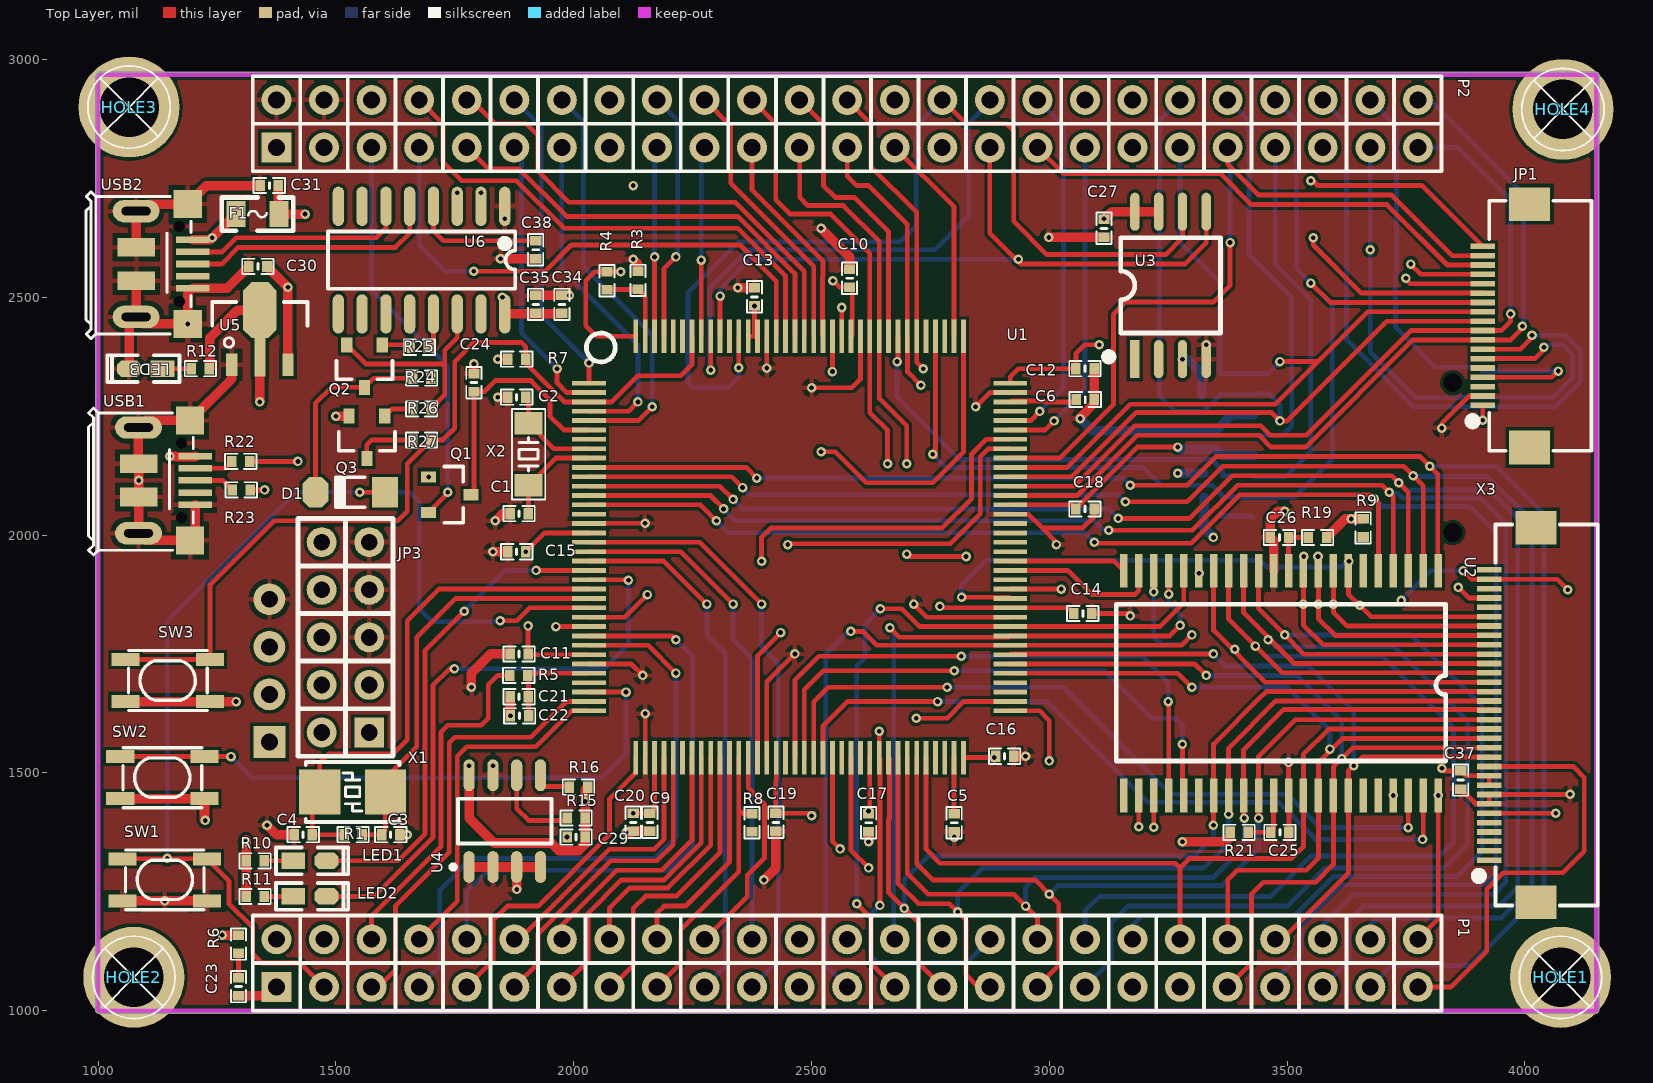
[diagram p0: Top Layer view]
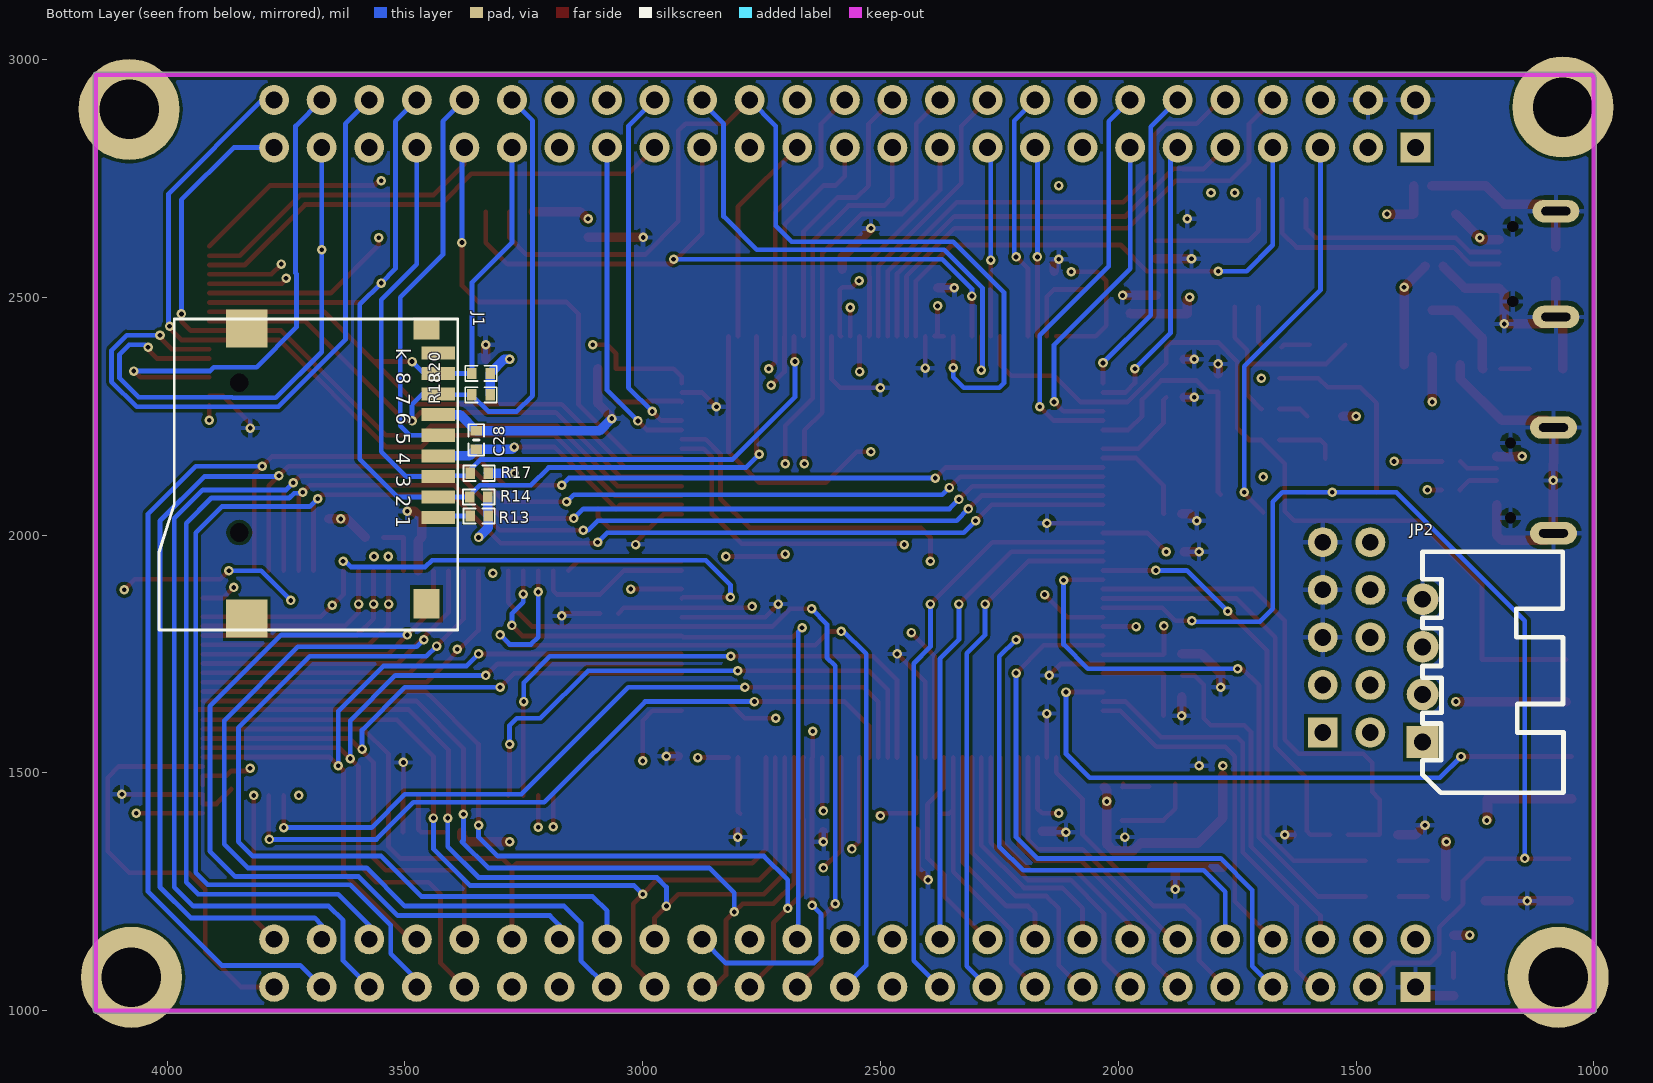
[diagram p1: Bottom Layer view, seen from below]
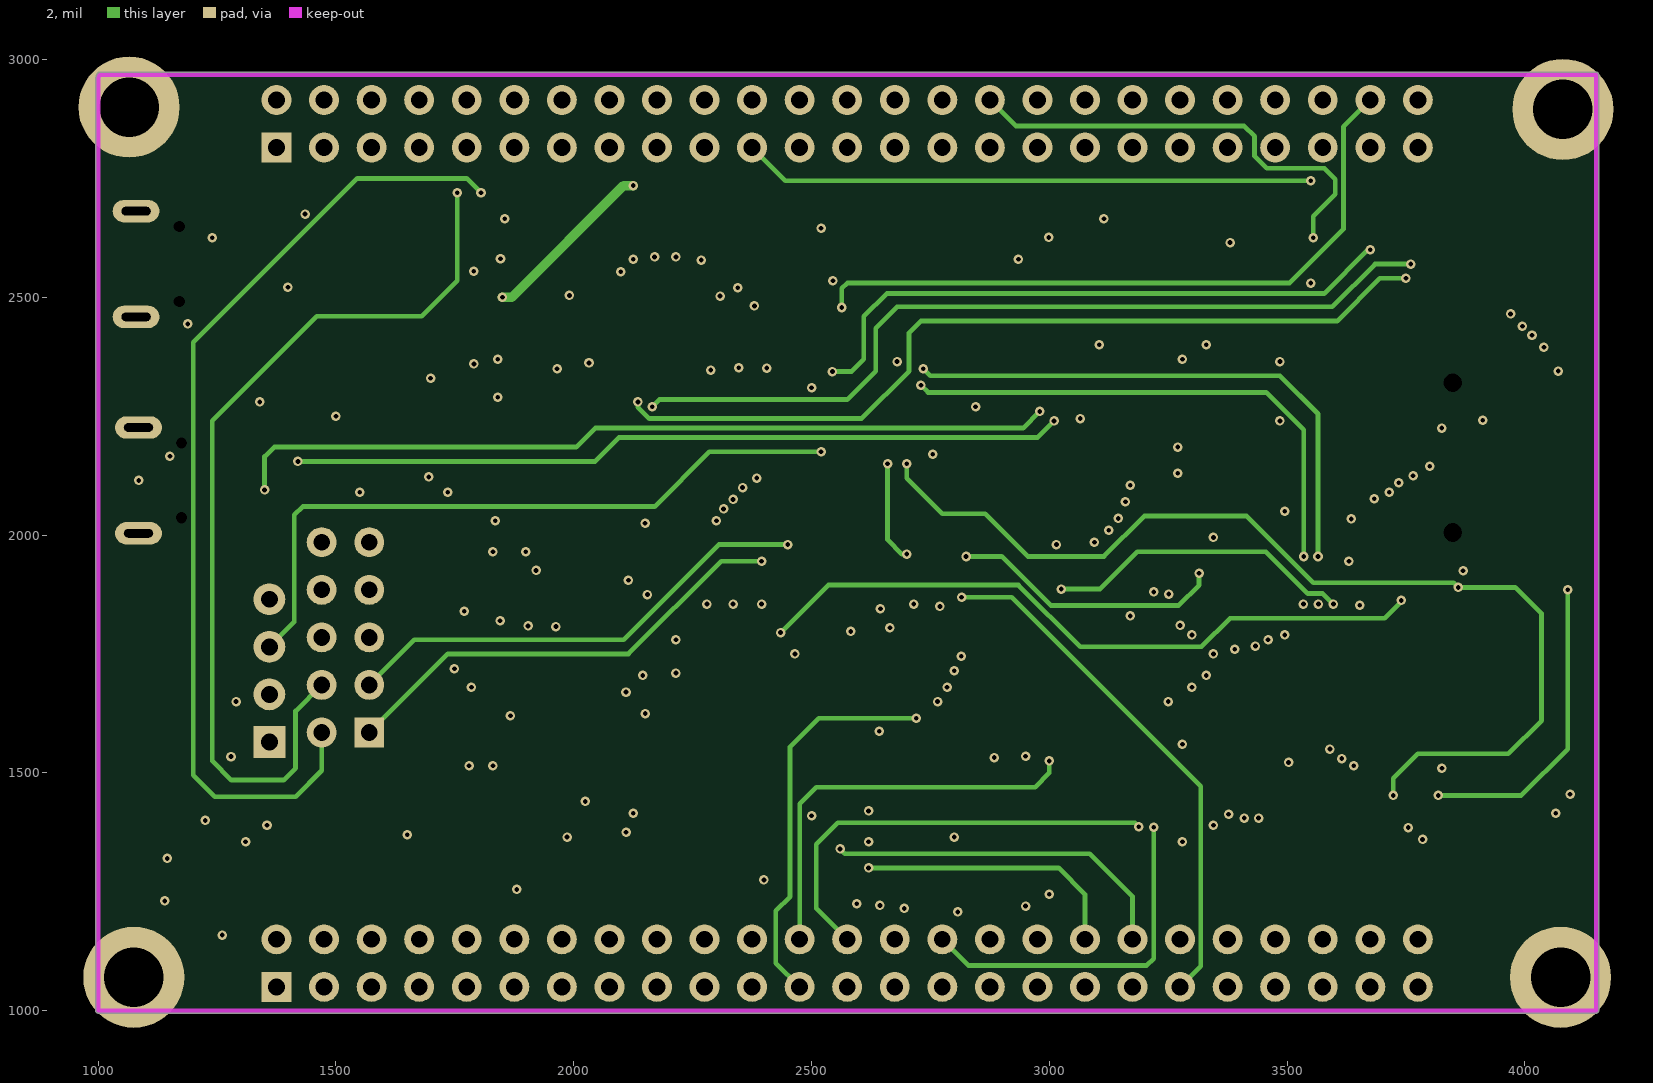
[diagram p2: 2]
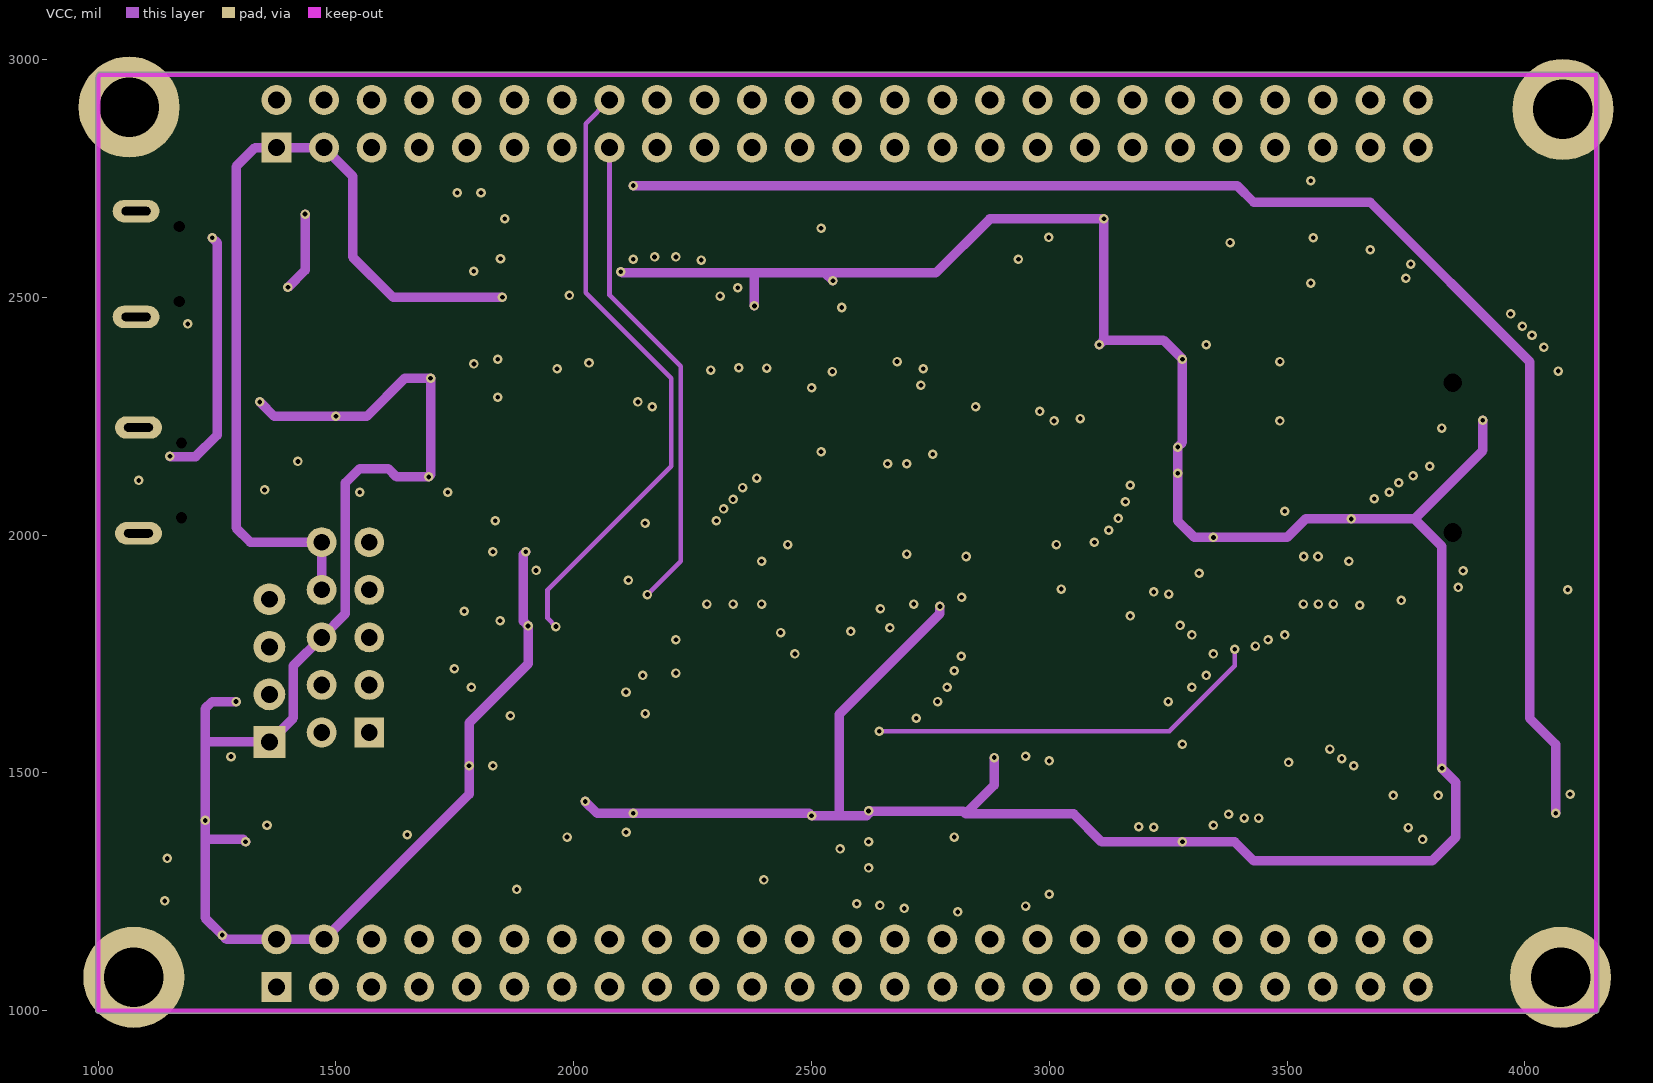
[diagram p3: VCC]
# Altium PCB MISC105440.PcbDoc (part 1 of 2)
Units mil, origin at the board's own origin, x right, y up, seen from the top; angles counter-clockwise.
Board outline 3160.03 x 1978.53 mil, 4 copper layers (Top Layer, 2, VCC, Bottom Layer), stack 30.634 mil thick; 91 components, 148 nets, 590 pads, 216 vias.

## Layer stack, top to bottom
Top Solder: solder mask 0.4, Solder Resist, Dk 3.5
Top Layer: signal copper 1.4
Dielectric 1: core 10, FR-4, Dk 4.2
2: signal copper 1.417
Dielectric 4: prepreg 5, Dk 4.2
VCC: signal copper 1.417
Dielectric 3: core 10, Dk 4.2
Bottom Layer: signal copper 1.4
Bottom Solder: solder mask 0.4, Solder Resist, Dk 3.5

## Board outline
1000,994.99 cw(c1000,1000) 994.99,1000 994.99,2960.15 cw(c1011.81,2960.15) 999.91,2972.05 cw(c1003.46,2968.5) 1003.46,2973.52 4149.61,2973.52 cw(c4149.61,2968.5) 4153.15,2972.05 cw(c4148.66,2967.55) 4155.02,2967.55 4155.02,1000 cw(c4150,1000) 4150,994.99

## Design rules (kind name [scope] priority, off if disabled: settings)
Clearance [All] p1: gap=7
HoleSize [All] p1: absolutevalues=TRUE maxlimit=99999 minlimit=1 maxpercent=80.000 minpercent=20.000
MinimumSolderMaskSliver [All] p1: minsoldermaskwidth=0
PolygonConnect [All] p1: connectstyle=Relief reliefconductorwidth=10 reliefentries=4 polygonreliefangle="90 Angle" airgapwidth=10
RoutingVias [All] p1: holewidth=28 width=50 viastyle="Through Hole" minholewidth=28 minwidth=50 maxholewidth=28 maxwidth=50
SilkToSilkClearance [All] p1: silktosilkclearance=0
SilkToSolderMaskClearance [IsPad] p1: minsilkscreentomaskgap=0 clearancetoexposedcopper=TRUE
SolderMaskExpansion [All] p1: expansion=4
Width [All] p1: maxlimit=30 minlimit=7 preferedwidth=7
26 further rules are at their usual default settings.

## Classes and differential pairs
component class Sheet1: C1 C2 C3 C4 C5 C6 C9 C10 C11 C12 C13 C14 C15 C16 C17 C18 C19 C20 C21 C22 C23 C24 JP1 JP2 P1 P2 Q1 R1 R3 R4 R5 R6 R7 R8 SW1 U1 X1 X2
component class Sheet2: C25 C26 C27 C28 C29 C30 C31 C34 C35 C37 C38 D1 F1 HOLE1 HOLE2 HOLE3 HOLE4 J1 JP3 LED1 LED2 LED3 Q2 Q3 R9 R10 R11 R12 R13 R14 R15 R16 R17 R18 R19 R20 R21 R22 R23 R24 R25 R26 R27 SW2 SW3 U2 U3 U4 U5 U6 USB1 USB2 X3

## Components (designator, comment, footprint, x,y, rotation, side; value= is the part's Value field where it differs from the comment)
C1 "10P" "C 0402" 1885,2045 r0 top
C2 "10P" "C 0402" 1880,2290 r0 top
C3 "22P" "C 0402" 1615,1370 r180 top
C4 "22P" "C 0402" 1431,1370 r0 top
C5 "225" "C 0402" 2800,1395 r270 top
C6 "225" "C 0402" 3075.59,2285 r0 top
C9 "104" "C 0402" 2160,1396 r90 top
C10 "104" "C 0402" 2580,2540 r270 top
C11 "104" "C 0402" 1885,1750 r0 top
C12 "104" "C 0402" 3075,2350 r180 top
C13 "104" "C 0402" 2380,2501 r270 top
C14 "104" "C 0402" 3070.59,1835 r180 top
C15 "104" "C 0402" 1880,1965 r0 top
C16 "104" "C 0402" 2906,1535 r180 top
C17 "104" "C 0402" 2620,1395 r90 top
C18 "104" "C 0402" 3075,2055 r180 top
C19 "104" "C 0402" 2425,1396 r90 top
C20 "104" "C 0402" 2125,1396 r90 top
C21 "10UF" "C 0402" 1885,1660 r180 top
C22 "104" "C 0402" 1886,1620 r180 top
C23 "104" "C 0402" 1295,1050.59 r270 top
C24 "104" "C 0402" 1790,2320.59 r270 top
C25 "10U" "C 0402" 3485,1375 r0 top
C26 "10U" "C 0402" 3484,1995 r180 top
C27 "104" "C 0402" 3115,2645 r270 top
C28 "104" "C 0402" 3350,2200 r270 bottom
C29 "104" "C 0402" 2005,1365 r0 top
C30 "22UF" "C 0402" 1336,2565 r0 top
C31 "104" "C 0402" 1360,2735 r0 top
C34 "10UF" "C 0402" 1975,2485 r90 top
C35 "104" "C 0402" 1920,2485 r90 top
C37 "104" "C 0402" 3865,1485 r90 top
C38 "104" "C 0402" 1920,2600 r90 top
D1 "1N4148" "MINI_MELF (LL34)" 1530,2090 r180 top
F1 "MSMD200-8V 2A" "FU 0805" 1335,2675 r0 top
HOLE1 "M3" "M3 5.4MM" 4075,1070 r0 top
HOLE2 "M3" "M3 5.4MM" 1075,1070 r0 top
HOLE3 "M3" "M3 5.4MM" 1065,2900 r0 top
HOLE4 "M3" "M3 5.4MM" 4080,2895 r0 top
J1 "TF_Card" "Micro SD" 3848.39,2162.76 r270 bottom
JP1 "FPC0.5-18P" "FPC0.5 2H-WS-18P" 4010,2440 r90 top
JP2 "SWD" XH2.54-WI-4P 1360,1715 r90 bottom
JP3 "Header 5X2" HDR2.54-LI-2x5P 1520,1785 r90 top
LED1 "Red" "LED 0603R" 1445,1314.74 r0 top
LED2 "Red" "LED 0603R" 1445,1240 r0 top
LED3 "Red" "LED 0603R" 1100,2350.26 r180 top
P1 "Header 25X2" HDR2.54-LI-2x25P 2325,1100 r0 top
P2 "Header 25X2" HDR2.54-LI-2x25P 2325,2865 r0 top
Q1 "BAT54C" SOT23-3L 1740,2085 r270 top
Q2 "SS8050" SOT23-3L 1560,2355 r180 top
Q3 "SS8550" SOT23-3L 1565,2205 r180 top
R1 "1M" "R 0402" 1536,1370 r180 top
R3 "0R" "R 0402" 2135,2535.59 r90 top
R4 "0R" "R 0402" 2070,2535 r90 top
R5 "10R" "R 0402" 1884.41,1705 r0 top
R6 "10K" "R 0402" 1295,1140 r90 top
R7 "10K" "R 0402" 1880,2370 r0 top
R8 "10K" "R 0402" 2375,1395 r90 top
R9 "10K" "R 0402" 3660,2015 r90 top
R10 "510" "R 0402" 1330,1315 r180 top
R11 "510" "R 0402" 1330,1240 r180 top
R12 "1K" "R 0402" 1215,2350 r0 top
R13 "47K" "R 0402" 3344,2040 r0 bottom
R14 "47K" "R 0402" 3345,2080 r0 bottom
R15 "4.7K" "R 0402" 2005,1405 r0 top
R16 "4.7K" "R 0402" 2010,1470 r0 top
R17 "47K" "R 0402" 3344,2130 r0 bottom
R18 "47K" "R 0402" 3340,2295 r0 bottom
R19 "2R" "R 0402" 3564,1995 r180 top
R20 "47K" "R 0402" 3340,2340 r0 bottom
R21 "2R" "R 0402" 3399,1375 r0 top
R22 "10R" "R 0402" 1300,2155 r0 top
R23 "10R" "R 0402" 1300.59,2095 r0 top
R24 "10K" "R 0402" 1680,2330 r180 top
R25 "1K" "R 0402" 1675.59,2395 r180 top
R26 "1K" "R 0402" 1680,2265 r180 top
R27 "1K" "R 0402" 1680,2200 r0 top
SW1 "3x6x5" "TSW SMD-3*4*2.5" 1140,1275 r0 top
SW2 "3x6x5" "TSW SMD-3*4*2.5" 1135,1490 r180 top
SW3 "3x6x5" "TSW SMD-3*4*2.5" 1146.42,1694.29 r180 top
U1 "STM32F407" "LQFP144 20X20_M" 2475,1975 r270 top
U2 "IS61LV51216" TSOP44_M 3817.93,1924.65 r270 top
U3 "W25Q128" SOP8W_L 3255,2525 r90 top
U4 "24C02C-E/ST" SOP8_L 1855,1398.54 r90 top
U5 "AS1117B" SOT89_L 1340,2370 r0 top
U6 "CH340G" SOP16 1855,2691.38 r270 top
USB1 "USB-DEVICE" USB-MICRO_B 1085,2115 r270 top
USB2 "USB-DEVICE" USB-MICRO_B 1080,2570 r270 top
X1 "8MHz" "OSC 5032-2P" 1535,1460 r180 top
X2 "32.768KHZ" "OSC 3215-2P" 1905,2170 r270 top
X3 "FPC0.5-32P" "FPC0.5 2H-WS-32P" 4023.31,1621.73 r90 top

## Footprints (in the part's own frame and the unit in brackets; to place one, negate y for a bottom-side part, rotate by r counter-clockwise, add the part's x,y. Pads: shape width x height; smd on the part's side, far side on the other; paste and mask are expansions set on the pad)
"C 0402" [mil] "无极性贴片电容"
  rect 20x23.62 smd mask+2: 1(-19,0) 2(19,0)
  silkscreen extent -33,-16 33,16, body extent -20,-10 20,10, height 20
"FPC0.5 2H-WS-18P" [mm] "长：13.2mm，宽：5.2mm，高：2mm"
  rect 1.8x2.2 smd: 0(-6.5,0) 0(6.5,0)
  rect 0.3x1.3 smd: 1(-4.25,2.497) 2(-3.75,2.497) 3(-3.25,2.497) 4(-2.75,2.497) 5(-2.25,2.497) 6(-1.75,2.497) 7(-1.25,2.497) 8(-0.75,2.497) 9(-0.25,2.497) 10(0.25,2.497) 11(0.75,2.497) 12(1.25,2.497) 13(1.75,2.497) 14(2.25,2.497) 15(2.75,2.497) 16(3.25,2.497) 17(3.75,2.497) 18(4.25,2.497)
  silkscreen extent -6.68,-3.3 6.68,3.23, body extent -6.6,-3.15 6.6,2.85, height 2
"FPC0.5 2H-WS-32P" [mm] "长：20.2mm，宽：5.2mm，高：2mm"
  rect 1.8x2.2 smd: 0(-10,0) 0(10,0)
  rect 0.3x1.3 smd: 1(-7.75,2.497) 2(-7.25,2.497) 3(-6.75,2.497) 4(-6.25,2.497) 5(-5.75,2.497) 6(-5.25,2.497) 7(-4.75,2.497) 8(-4.25,2.497) 9(-3.75,2.497) 10(-3.25,2.497) 11(-2.75,2.497) 12(-2.25,2.497) 13(-1.75,2.497) 14(-1.25,2.497) 15(-0.75,2.497) 16(-0.25,2.497) 17(0.25,2.497) 18(0.75,2.497) 19(1.25,2.497) 20(1.75,2.497) 21(2.25,2.497) 22(2.75,2.497) 23(3.25,2.497) 24(3.75,2.497) 25(4.25,2.497) 26(4.75,2.497) 27(5.25,2.497) 28(5.75,2.497) 29(6.25,2.497) 30(6.75,2.497) 31(7.25,2.497) 32(7.75,2.497)
  silkscreen extent -10.18,-3.3 10.17,3.23, body extent -10.1,-3.15 10.1,2.85, height 2
"FU 0805" [mil] "贴片保险丝"
  rect 40x55 smd: 1(-45,0) 2(45,0)
  silkscreen extent -75,-35 75,35, body extent -39,-24 39,24, height 20
HDR2.54-LI-2x5P [mm] "双排排针，5x2脚"
  rect 1.6x1.6 hole 0.9: 1(-5.08,-1.27)
  round 1.6 hole 0.9: 2(-5.08,1.27) 3(-2.54,-1.27) 4(-2.54,1.27) 5(0,-1.27) 6(0,1.27) 7(2.54,-1.27) 8(2.54,1.27) 9(5.08,-1.27) 10(5.08,1.27)
  silkscreen extent -6.35,-2.54 6.35,2.54, body extent -6.35,-2.54 6.35,2.54, height 8.5
HDR2.54-LI-2x25P [mm] "双排排针，25x2脚"
  rect 1.6x1.6 hole 0.9: 1(-24.13,-1.27)
  round 1.6 hole 0.9: 2(-24.13,1.27) 3(-21.59,-1.27) 4(-21.59,1.27) 5(-19.05,-1.27) 6(-19.05,1.27) 7(-16.51,-1.27) 8(-16.51,1.27) 9(-13.97,-1.27) 10(-13.97,1.27) 11(-11.43,-1.27) 12(-11.43,1.27) 13(-8.89,-1.27) 14(-8.89,1.27) 15(-6.35,-1.27) 16(-6.35,1.27) 17(-3.81,-1.27) 18(-3.81,1.27) 19(-1.27,-1.27) 20(-1.27,1.27) 21(1.27,-1.27) 22(1.27,1.27) 23(3.81,-1.27) 24(3.81,1.27) 25(6.35,-1.27) 26(6.35,1.27) 27(8.89,-1.27) 28(8.89,1.27) 29(11.43,-1.27) 30(11.43,1.27) 31(13.97,-1.27) 32(13.97,1.27) 33(16.51,-1.27) 34(16.51,1.27) 35(19.05,-1.27) 36(19.05,1.27) 37(21.59,-1.27) 38(21.59,1.27) 39(24.13,-1.27) 40(24.13,1.27) 41(26.67,-1.27) 42(26.67,1.27) 43(29.21,-1.27) 44(29.21,1.27) 45(31.75,-1.27) 46(31.75,1.27) 47(34.29,-1.27) 48(34.29,1.27) 49(36.83,-1.27) 50(36.83,1.27)
  silkscreen extent -25.4,-2.54 38.1,2.54, body extent -25.4,-2.54 38.1,2.54, height 8.5
"LED 0603R" [mil] "红色0603LED"
  rect 50x35 smd: 1(-35,0.26)
  oct 50x35 smd: 2(35,0.26)
  silkscreen extent -71,-28 81,28, body extent -31,-16 31,16, height 18
"LQFP144 20X20_M" [mm] "144脚，体宽20x20mm，脚距0.5mm"
  rect 0.254x1.8 smd: 1(-8.75,-11.25) 2(-8.25,-11.25) 3(-7.75,-11.25) 4(-7.25,-11.25) 5(-6.75,-11.25) 6(-6.25,-11.25) 7(-5.75,-11.25) 8(-5.25,-11.25) 9(-4.75,-11.25) 10(-4.25,-11.25) 11(-3.75,-11.25) 12(-3.25,-11.25) 13(-2.75,-11.25) 14(-2.25,-11.25) 15(-1.75,-11.25) 16(-1.25,-11.25) 17(-0.75,-11.25) 18(-0.25,-11.25) 19(0.25,-11.25) 20(0.75,-11.25) 21(1.25,-11.25) 22(1.75,-11.25) 23(2.25,-11.25) 24(2.75,-11.25) 25(3.25,-11.25) 26(3.75,-11.25) 27(4.25,-11.25) 28(4.75,-11.25) 29(5.25,-11.25) 30(5.75,-11.25) 31(6.25,-11.25) 32(6.75,-11.25) 33(7.25,-11.25) 34(7.75,-11.25) 35(8.25,-11.25) 36(8.75,-11.25) 73(8.75,11.25) 74(8.25,11.25) 75(7.75,11.25) 76(7.25,11.25) 77(6.75,11.25) 78(6.25,11.25) 79(5.75,11.25) 80(5.25,11.25) 81(4.75,11.25) 82(4.25,11.25) 83(3.75,11.25) 84(3.25,11.25) 85(2.75,11.25) 86(2.25,11.25) 87(1.75,11.25) 88(1.25,11.25) 89(0.75,11.25) 90(0.25,11.25) 91(-0.25,11.25) 92(-0.75,11.25) 93(-1.25,11.25) 94(-1.75,11.25) 95(-2.25,11.25) 96(-2.75,11.25) 97(-3.25,11.25) 98(-3.75,11.25) 99(-4.25,11.25) 100(-4.75,11.25) 101(-5.25,11.25) 102(-5.75,11.25) 103(-6.25,11.25) 104(-6.75,11.25) 105(-7.25,11.25) 106(-7.75,11.25) 107(-8.25,11.25) 108(-8.75,11.25)
  rect 1.8x0.254 smd: 37(11.25,-8.75) 38(11.25,-8.25) 39(11.25,-7.75) 40(11.25,-7.25) 41(11.25,-6.75) 42(11.25,-6.25) 43(11.25,-5.75) 44(11.25,-5.25) 45(11.25,-4.75) 46(11.25,-4.25) 47(11.25,-3.75) 48(11.25,-3.25) 49(11.25,-2.75) 50(11.25,-2.25) 51(11.25,-1.75) 52(11.25,-1.25) 53(11.25,-0.75) 54(11.25,-0.25) 55(11.25,0.25) 56(11.25,0.75) 57(11.25,1.25) 58(11.25,1.75) 59(11.25,2.25) 60(11.25,2.75) 61(11.25,3.25) 62(11.25,3.75) 63(11.25,4.25) 64(11.25,4.75) 65(11.25,5.25) 66(11.25,5.75) 67(11.25,6.25) 68(11.25,6.75) 69(11.25,7.25) 70(11.25,7.75) 71(11.25,8.25) 72(11.25,8.75) 109(-11.25,8.75) 110(-11.25,8.25) 111(-11.25,7.75) 112(-11.25,7.25) 113(-11.25,6.75) 114(-11.25,6.25) 115(-11.25,5.75) 116(-11.25,5.25) 117(-11.25,4.75) 118(-11.25,4.25) 119(-11.25,3.75) 120(-11.25,3.25) 121(-11.25,2.75) 122(-11.25,2.25) 123(-11.25,1.75) 124(-11.25,1.25) 125(-11.25,0.75) 126(-11.25,0.25) 127(-11.25,-0.25) 128(-11.25,-0.75) 129(-11.25,-1.25) 130(-11.25,-1.75) 131(-11.25,-2.25) 132(-11.25,-2.75) 133(-11.25,-3.25) 134(-11.25,-3.75) 135(-11.25,-4.25) 136(-11.25,-4.75) 137(-11.25,-5.25) 138(-11.25,-5.75) 139(-11.25,-6.25) 140(-11.25,-6.75) 141(-11.25,-7.25) 142(-11.25,-7.75) 143(-11.25,-8.25) 144(-11.25,-8.75)
  silkscreen extent -11.43,-11.39 -9.88,-9.84, body extent -11,-11 11,11, height 1.45
"M3 5.4MM" [mm] "M3螺丝孔，"
  round 5.4 hole 3.175: 0(0,0)
  silkscreen extent -2.2,-2.2 2.2,2.2
"Micro SD" [mm]
  round 0.85 hole 1 unplated: 0(-4,0) 0(4,0)
  rect 0.7x1.8 smd: 1(3.2,10.627) 2(2.1,10.627) 3(1,10.627) 4(-0.1,10.627) 5(-1.2,10.627) 6(-2.3,10.627) 7(-3.4,10.627) 8(-4.5,10.627) 9(-5.6,10.627)
  rect 2.032x2.2 smd: 10(-6.9,0.4) 10(8.6,0.4)
  rect 1.2x1.4 smd: 10(-6.9,10)
  rect 1.6x1.4 smd: 10(7.8,10)
  silkscreen extent -7.4,-4.28 9.2,11.67, body extent -7.05,-4 8.95,11.25, height 2
"MINI_MELF (LL34)" [mm] "1.5*3.4mm(直径，脚距）"
  rect 1.37x1.62 smd: 1(-1.855,0)
  oct 1.37x1.62 smd: 2(1.855,0)
  silkscreen extent -0.76,-0.8 0.78,0.8, body extent -1.7,-0.75 1.7,0.75, height 1.5
"OSC 3215-2P" [mm] "3.2*1.5*0.6mm(长宽高)"
  rect 1.2x1.5 smd: 1(-1.65,0) 2(1.65,0)
  silkscreen extent -2.41,-0.89 2.41,0.89, body extent -1.6,-0.75 1.6,0.75, height 0.61
"OSC 5032-2P" [mm] "5mm*3.2mm*0.8mm(长*宽*高)"
  rect 2.2x2.4 smd: 1(-1.75,0) 2(1.75,0)
  silkscreen extent -2.5,-1.6 2.5,1.6, body extent -2.5,-1.6 2.5,1.6, height 0.86
"R 0402" [mil] "1/16W贴片电阻"
  rect 20x23.62 smd mask+2: 1(-19,0) 2(19,0)
  silkscreen extent -33,-16 33,16, body extent -20,-10 20,10, height 12
SOP8_L [mm] "SOIC, 8-Leads, Body 4.9x3.9mm, Pitch 1.27mm, IPC High Density"
  oval 1.7x0.6 smd: 1(-2.45,1.905) 2(-2.45,0.635) 3(-2.45,-0.635) 4(-2.45,-1.905) 5(2.45,-1.905) 6(2.45,-0.635) 7(2.45,0.635) 8(2.45,1.905)
  silkscreen extent -2.57,-2.5 1.2,2.88, body extent -2,-2.5 2,2.5, height 1.75
SOP8W_L [mil] "5.3*8.3*1.8mm（长宽高）"
  rect 80x19.68 smd: 1(-155,75)
  oval 80x19.68 smd: 2(-155,25) 3(-155,-25) 4(-155,-75) 5(155,-75) 6(155,-25) 7(155,25) 8(155,75)
  silkscreen extent -156,-105 100,136, body extent -155,-104 155,104, height 75
SOP16 [mm]
  oval 2.1x0.6 smd: 1(0,0) 2(0,-1.27) 3(0,-2.54) 4(0,-3.81) 5(0,-5.08) 6(0,-6.35) 7(0,-7.62) 8(0,-8.89) 9(5.75,-8.89) 10(5.75,-7.62) 11(5.75,-6.35) 12(5.75,-5.08) 13(5.75,-3.81) 14(5.75,-2.54) 15(5.75,-1.27) 16(5.75,0)
  silkscreen extent 1.35,-9.45 4.4,0.56, body extent -0.04,-9.45 5.97,0.56, height 1.9
SOT23-3L [mm] "3x1.3x1mm(长宽高)"
  rect 0.6x0.8 smd: 1(-0.95,-1.143) 2(0.95,-1.143) 3(0,1.125)
  silkscreen extent -1.5,-0.3 1.5,0.7, body extent -1.5,-1.2 1.5,1.2, height 1.05
SOT89_L [mm] "4.6x4.3x1.6mm(长宽高)"
  rect 0.6x1.2 smd: 1(-1.5,-0.303) 3(1.5,-0.303)
  rect 0.6x2.1 smd: 2(0,0.127)
  oct 1.8x3 smd: 2(0,2.616)
  silkscreen extent -2.54,0.64 2.54,3.05, body extent -2.31,-0.63 2.29,3.67, height 1.6
TSOP44_M [mm]
  rect 1.8x0.4 smd: 1(-0.009,0.001) 2(-0.009,-0.799) 3(-0.009,-1.599) 4(-0.009,-2.399) 5(-0.009,-3.199) 6(-0.009,-3.999) 7(-0.009,-4.799) 8(-0.009,-5.599) 9(-0.009,-6.399) 10(-0.009,-7.199) 11(-0.009,-7.999) 12(-0.009,-8.799) 13(-0.009,-9.599) 14(-0.009,-10.399) 15(-0.009,-11.199) 16(-0.009,-11.999) 17(-0.009,-12.799) 18(-0.009,-13.599) 19(-0.009,-14.399) 20(-0.009,-15.199) 21(-0.009,-15.999) 22(-0.009,-16.799) 23(11.991,-16.799) 24(11.991,-15.999) 25(11.991,-15.199) 26(11.991,-14.399) 27(11.991,-13.599) 28(11.991,-12.799) 29(11.991,-11.999) 30(11.991,-11.199) 31(11.991,-10.399) 32(11.991,-9.599) 33(11.991,-8.799) 34(11.991,-7.999) 35(11.991,-7.199) 36(11.991,-6.399) 37(11.991,-5.599) 38(11.991,-4.799) 39(11.991,-3.999) 40(11.991,-3.199) 41(11.991,-2.399) 42(11.991,-1.599) 43(11.991,-0.799) 44(11.991,0.001)
  silkscreen extent 1.77,-17.2 10.16,0.4, body extent 0.1,-17.55 11.86,0.66, height 1.3
"TSW SMD-3*4*2.5" [mm] "3*4*2.5mm"
  rect 1.5x0.7 smd: 1(-2.25,1.125) 1(2.25,1.125) 2(-2.25,-1.125) 2(2.25,-1.125)
  silkscreen extent -2.1,-1.6 2.1,1.6
USB-MICRO_B [mm] "micro型USB ，5.9*8.2*2.5mm"
  rect 0.35x1.8 smd: 1(-1.295,3.021) 2(-0.648,3.021) 3(0,3.021) 4(0.648,3.021) 5(1.295,3.021)
  rect 1.5x1.5 smd: 5(-3.2,2.754) 5(3.2,2.754)
  oval 1.2x2.5 hole 0.45 slot 1.55 at 90 deg: 5(-2.825,-0.006) 5(2.825,-0.006)
  round 0 hole 0.6 unplated: 5(-2,2.294) 5(2,2.294)
  rect 1x2 smd: 5(-0.889,0.01) 5(0.889,0.01)
  silkscreen extent -3.86,-2.67 3.99,2.92, body extent -4,-2.72 4,3.36, height 2.8
XH2.54-WI-4P [mm] "接插件，4P"
  rect 1.7x1.7 hole 0.9: 1(-3.81,0)
  round 1.7 hole 0.9: 2(-1.27,0) 3(1.27,0) 4(3.81,0)
  silkscreen extent -6.53,-7.53 6.35,0, body extent -6.31,-7.35 6.31,0.35, height 5.73

## Part data
C1 C2 C3 C4 C5 C6 C9 C10 C11 C12 C13 C14 C15 C16 C17 C18 C19 C20 C21 C22 C23 C24 C25 C26 C27 C28 C29 C30 C31 C34 C35 C38: library part C, "SMD capacitor"
C37: library part C, "Non-polar SMD capacitor"
D1: "Switching diode"
F1: library part FU, "SMD fuse"
HOLE1 HOLE2 HOLE3 HOLE4: "Copper pillar hole"
J1: "TF card socket"
JP1: library part FPC-18P, "FPC connector"
JP2: library part "Header 4", "4P connector"
JP3: "5*2P connector"
LED1 LED2 LED3: library part LED-SMD, "SMD LED"
P1 P2: "Header, 25-Pin, Dual row"
Q1: "SMD Schottky diode"
Q2: library part 8050-SMD, "RF amplifier, NPN type"
Q3: library part 8550-SMD, "RF amplifier, PNP type"
R1 R3 R4 R5 R6 R7 R8 R9 R10 R11 R12 R13 R14 R15 R16 R17 R18 R19 R20 R21 R22 R23 R24 R25 R26 R27: library part R, "SMD resistor"
SW1 SW2 SW3: library part "TSW 3x6", "3x6 tactile switch"
U2: "Static RAM"
U4: "2Kbit, 400kHz, 5V, I2C Serial EEPROM, 8-Pin TSSOP, Extended Temperature"
U5: library part AMS1117, "Three-terminal voltage regulator"
U6: "USB2UART"
USB1 USB2: library part USB-5P, "Micro USB receptacle"
X1 X2: library part XTAL-2P, "2-pin passive crystal oscillator"
X3: library part FPC-32P, "FPC connector"

## Via types
v1: diameter 20, hole 10, Top Layer to Bottom Layer, 216 vias

## Nets (pads, with @x,y where several pads share a name; then routed paths per layer and width w, separated by ;. In a path a pad name is that pad's centre, name@x,y a point inside that pad or via, vN(x,y) a via of type N, cw(c..) or ccw(c..) an arc to the next point about the centre after c; other vN are vias at no path point)
BOOT0: R7.2 R27.2 SW3.2 U1.3 U1.138 | length 1863.7
  Top Layer w10: SW3.2@1057.83,1738.58 SW3.2@1235,1738.58 1235,1895 1370,2030 1630,2030 1650,2050 1650,2150.22 1699,2199.22 R27.2@1699,2200 1725,2200 1750,2225 1750,2365 1790,2405 1890,2405 1899,2396 R7.2@1899,2370 1899,2361 1979.88,2280.12 U1.3@2032.09,2280.12 2080.12,2280.12 2135,2335 2225,2335 2248.62,2358.62 U1.138@2248.62,2417.91
BOOT1: P1.17 R8.2 U1.48 | length 585
  Top Layer w10: P1.17@2175,1050 2225,1100 2225,1170 2347.05,1292.05 2347.05,1422.95 ; U1.48@2347.05,1532.09 2347.05,1422.95 ; R8.2@2375,1414 2356,1414 2347.05,1422.95
CH340_D+: U6.5 USB2.3 | length 554.4
  Top Layer w10: USB2.3@1198.94,2570 1260,2570 1295,2605 1625,2605 1655,2635 U6.5@1655,2691.38 U6.5@1655,2706.38
CH340_D-: U6.6 USB2.2 | length 487.9
  Top Layer w10: USB2.2@1198.94,2595.5 1260.5,2595.5 1290,2625 1585,2625 1605,2645 U6.6@1605,2691.38 U6.6@1605,2706.38
DCMI_D0: JP1.8 P2.50 U1.96 | length 1834.9
  Top Layer w10: U1.96@2917.91,2083.27 3058.27,2083.27 3185,2210 3440.96,2210 3465.96,2185 3539.04,2185 3764.51,2410.47 JP1.8@3911.69,2410.47 3970.47,2410.47 3995,2435 v1(3995,2439)
  Bottom Layer w10: P2.50@3775,2915 3800,2915 3997,2718 3997,2437 v1(3995,2439)
DCMI_D1: JP1.9 P2.49 U1.97 | length 1708
  Top Layer w10: U1.97@2917.91,2102.95 3052.95,2102.95 3180,2230 3445,2230 3465,2210 3540,2210 3760.16,2430.16 JP1.9@3911.69,2430.16 3950.16,2430.16 3970,2450 v1(3970,2465)
  Bottom Layer w10: P2.49@3775,2815 3860,2815 3970,2705 v1(3970,2465)
DCMI_D2: J1.7 JP1.10 P2.40 R18.2 U1.98 | length 2110.7
  Top Layer w10: U1.98@2917.91,2122.64 3047.64,2122.64 3183,2258 3467,2258 v1(3485,2240) 3500,2240 3709.84,2449.84 JP1.10@3911.69,2449.84
  Bottom Layer w10: P2.40@3275,2915 3231.5,2871.5 3231.5,2293.5 3265,2260 3324.78,2260 3359,2294.22 R18.2@3359,2295 3428.39,2295 J1.7@3430,2296.61 3463.39,2296.61 3485,2275 v1(3485,2240)
DCMI_D3: J1.8 JP1.11 P2.39 R20.2 U1.99 | length 1855.4
  Top Layer w10: U1.99@2917.91,2142.32 3037.32,2142.32 3170,2275 3475,2275 3564.76,2364.76 ; v1(3485,2365) 3564.53,2365 3564.76,2364.76 ; JP1.11@3911.69,2469.53 3669.53,2469.53 3564.76,2364.76
  Bottom Layer w10: P2.39@3275,2815 3275,2615 3359,2531 R20.2@3359,2340 3359.08,2339.92 J1.8@3430,2339.92 3459.92,2339.92 v1(3485,2365)
DCMI_D4: J1.2 JP1.12 P2.44 R14.2 U1.112 | length 2345.8
  Top Layer w10: v1(2755,2170) 2760.43,2164.57 U1.112@2760.43,2417.91 ; v1(3550,2530) 3590.79,2489.21 JP1.12@3911.69,2489.21
  Bottom Layer w10: v1(2755,2170) 2783,2142 3198,2142 3235,2105 3342.78,2105 3364,2083.78 R14.2@3364,2080 ; 3375.08,2080.08 J1.2@3430,2080.08 3515.08,2080.08 3595,2160 3595,2485 v1(3550,2530) 3520,2560 3520,2870.01 P2.44@3475,2915
DCMI_D5: JP1.13 P2.32 U1.136 | length 2490.9
  Top Layer w10: v1(2287.99,2347.01) U1.136@2287.99,2417.91 ; v1(3555,2625) 3555,2610 3656.1,2508.9 JP1.13@3911.69,2508.9
  2 w10: P2.32@2875,2915 2930,2860 3410,2860 3431.51,2838.49 3431.51,2796.99 3456.99,2771.51 3578.49,2771.51 3601.5,2748.5 3601.5,2716.5 3555,2670 v1(3555,2625)
  Bottom Layer w10: v1(2287.99,2347.01) 2285.68,2349.32 2285.68,2519.72 2365.96,2600 2760,2600 2830,2670 2830,2865 2875,2910 P2.32@2875,2915
DCMI_D6: JP1.14 P2.13 U1.4 | length 2685.4
  Top Layer w10: U1.4@2032.09,2260.43 2115.43,2260.43 v1(2135,2280) ; v1(3750,2540) 3750,2537.16 3758.58,2528.58 JP1.14@3911.69,2528.58
  2 w10: v1(2135,2280) 2135,2268.89 2158.89,2245 2605,2245 2705,2345 2705,2425 2730,2450 3605,2450 3695,2540 v1(3750,2540)
  Bottom Layer w10: P2.13@1975,2815 1975,2560 2135,2400 v1(2135,2280)
DCMI_D7: JP1.15 P2.14 U1.5 | length 2802.1
  Top Layer w10: U1.5@2032.09,2240.75 2135.75,2240.75 v1(2165,2270) ; v1(3760,2570) 3760,2568.89 3780.62,2548.27 JP1.15@3911.69,2548.27
  2 w10: v1(2165,2270) 2180,2285 2575,2285 2635,2345 2635,2435 2680,2480 3595,2480 3685,2570 v1(3760,2570)
  Bottom Layer w10: P2.14@1975,2915 2020,2870 2020,2565 2165,2420 v1(2165,2270)
DCMI_HREF: P1.12 U1.40 | length 573.9
  Top Layer w10: P1.12@1875,1150 1885,1150 2074.57,1339.57 2169.57,1339.57 2189.57,1359.57 U1.40@2189.57,1532.09
DCMI_PCLK: JP1.16 P2.33 | length 1039
  Top Layer w10: P2.33@2975,2815 3030,2760 3360,2760 3425,2695 3710,2695 3837.05,2567.95 JP1.16@3911.69,2567.95
DCMI_PWDN: JP1.18 P2.21 U1.124 | length 2082.6
  Top Layer w10: P2.21@2375,2815 2375,2725 2524.21,2575.79 2524.21,2545.33 2523,2544.11 2523,2419.13 U1.124@2524.21,2417.91 ; v1(3550,2745) 3555,2745 3565,2735 3784.02,2735 JP1.18@3911.69,2607.32
  2 w10: P2.21@2375,2815 2445,2745 v1(3550,2745)
DCMI_RESET: JP1.7 P2.46 | length 1402.9
  Top Layer w10: JP1.7@3911.69,2390.79 3990.79,2390.79 4020,2420 v1(4015,2420)
  Bottom Layer w10: P2.46@3575,2915 3625,2865.01 3625,2410.96 3765.96,2270 4064.04,2270 4117,2322.96 4117,2388 4084.82,2420.18 4084.63,2420 v1(4015,2420)
DCMI_SCL: JP1.4 P2.48 U1.122 | length 2547.8
  Top Layer w10: U1.122@2563.58,2417.91 v1(2563.58,2478.58) ; JP1.4@3911.69,2331.73 4056.73,2331.73 v1(4070,2345)
  2 w10: v1(2563.58,2478.58) 2563.58,2518.58 2575,2530 3505,2530 3618.5,2643.5 3618.5,2858.5 P2.48@3675,2915
  Bottom Layer w10: P2.48@3675,2915 3730,2860.01 3730,2551.11 3728,2549.11 3728,2437 3812,2353 3902,2353 3910,2345 v1(4070,2345)
DCMI_SDA: JP1.6 P2.47 U1.123 | length 2537.5
  Top Layer w10: v1(2543.9,2343.9) U1.123@2543.9,2417.91 ; JP1.6@3911.69,2371.1 4021.1,2371.1 4040,2390 v1(4040,2395)
  2 w10: v1(2543.9,2343.9) 2583.9,2343.9 2610,2370 2610,2460 2658,2508 3578,2508 3670,2600 v1(3675,2600)
  Bottom Layer w10: P2.47@3675,2815 3675,2385 3771.45,2288.55 3861.51,2288.55 3862.96,2290 4060,2290 4100,2330 4100,2380 4080,2400 4045,2400 v1(4040,2395)
DCMI_VSYNC: P2.19 U1.137 | length 399.9
  Top Layer w10: U1.137@2268.31,2417.91 v1(2268.31,2578.31)
  Bottom Layer w10: v1(2268.31,2578.31) 2268.31,2808.31 P2.19@2275,2815
DCMI_XCLK: JP1.17 P2.41 U1.100 | length 1667.2
  Top Layer w10: U1.100@2917.91,2162.01 3022.01,2162.01 3135,2275 3135,2465 3160,2490 3345,2490 3380,2525 v1(3380,2615) ; P2.41@3375,2815 3375,2780 3440,2715 3720,2715 3847.36,2587.64 JP1.17@3911.69,2587.64
  Bottom Layer w10: P2.41@3375,2815 3380,2810.01 v1(3380,2615)
F_CS: U3.1
FSMC_A0: P1.47 U1.10 U2.1 | length 3568.9
  Top Layer w10: U1.10@2032.09,2142.32 2362.68,2142.32 v1(2385,2120) ; v1(3170,2105) 3290,2105 3350,2165 3780,2165 v1(3800,2145) 3816.7,2128.3 3816.7,1925 U2.1@3817.95,1925
  Bottom Layer w10: v1(2385,2120) 3155,2120 v1(3170,2105) ; P1.47@3675,1050 3720,1095 3885,1095 4040,1250 4040,2045 3940,2145 v1(3800,2145)
FSMC_A1: P1.48 U1.11 U2.2 | length 3465.4
  Top Layer w10: U1.11@2032.09,2122.64 2332.36,2122.64 v1(2355,2100) ; v1(3160,2070) 3290,2070 3365,2145 3745,2145 v1(3765,2125) 3786.46,2103.54 U2.2@3786.46,1925
  Bottom Layer w10: v1(2355,2100) 2370,2085 3145,2085 v1(3160,2070) ; P1.48@3675,1150 3675,1180 3690,1195 3950,1195 4015,1260 4015,2030 3922,2123 3767,2123 v1(3765,2125)
FSMC_A2: P1.45 U1.12 U2.3 | length 3570.7
  Top Layer w10: U1.12@2032.09,2102.95 2307.05,2102.95 v1(2335,2075) ; v1(3145,2035) 3295,2035 3385,2125 3720,2125 v1(3735,2110) 3754.96,2090.04 U2.3@3754.96,1925
  Bottom Layer w10: v1(2335,2075) 2355,2055 3125,2055 v1(3145,2035) ; P1.45@3575,1050 3630,1105 3630,1190 3660,1220 3945,1220 3985,1260 3985,2035 3925,2095 3750,2095 v1(3735,2110)
FSMC_A3: P1.46 U1.13 U2.4 | length 3406.5
  Top Layer w10: U1.13@2032.09,2083.27 2286.73,2083.27 v1(2315,2055) ; v1(3125,2010) 3300.96,2010 3395.96,2105 3700,2105 v1(3715,2090) 3723.47,2081.53 U2.4@3723.47,1925
  Bottom Layer w10: v1(2315,2055) 2340,2030 3095,2030 3115,2010 v1(3125,2010) ; P1.46@3575,1150 3575,1180 3640,1245 3935,1245 3960,1270 3960,2025 3907,2078 3742.96,2078 3732.96,2088 3717,2088 v1(3715,2090)
FSMC_A4: P1.43 U1.14 U2.5 | length 3495
  Top Layer w10: U1.14@2032.09,2063.58 2266.42,2063.58 v1(2300,2030) ; v1(3095,1985) 3097,1983 3298,1983 3400,2085 3675,2085 v1(3683.49,2076.51) 3691.97,2068.03 U2.5@3691.97,1925
  Bottom Layer w10: v1(2300,2030) 2325,2005 3075,2005 v1(3095,1985) ; P1.43@3475,1050 3475,1065 3530,1120 3530,1180 3615,1265 3915,1265 3940,1290 3940,2005 3885,2060 3700,2060 v1(3683.49,2076.51)
FSMC_A5: P1.26 U2.24 | length 992.5
  Top Layer w10: v1(3188.03,1386.97) U2.24@3188.03,1452.56
  2 w10: P1.26@2575,1150 2510,1215 2510,1350 2555,1395 3180,1395 v1(3188.03,1386.97)
FSMC_A6: P1.50 U1.50 U2.44 X3.31 | length 3092.9
  Top Layer w10: U1.50@2386.42,1532.09 2386.42,1746.42 v1(2435,1795) ; P1.50@3775,1150 3817.95,1192.95 v1(3817.95,1452.56) ; v1(3870,1925) 3887.83,1907.17 X3.31@3925,1907.17 4067.83,1907.17 v1(4090,1885)
  2 w10: v1(2435,1795) 2535,1895 2935,1895 3065,1765 3320,1765 3380,1825 3705,1825 3740,1860 v1(3740,1862.5) v1@3740,1865 ; v1(3817.95,1452.56) 3992.56,1452.56 4090,1550 v1(4090,1885)
  Bottom Layer w10: v1(3740,1862.5) 3802.5,1925 v1(3870,1925) v1@3875,1925
FSMC_A7: P1.30 U2.25 | length 816.4
  Top Layer w10: v1(3219.53,1385.47) U2.25@3219.53,1452.56
  2 w10: P1.30@2775,1150 2830,1095 3205,1095 3219.53,1109.53 v1(3219.53,1385.47)
FSMC_A8: U1.54 U2.26 | length 1229.2
  Top Layer w10: U1.54@2465.16,1532.09 2465.16,1695.16 2515,1745 v1(2815,1745) ; v1(3250,1650) 3251.02,1648.98 U2.26@3251.02,1452.56
  Bottom Layer w10: v1(2815,1745) 3195,1745 3250,1690 v1(3250,1650)
FSMC_A9: U1.55 U2.27 | length 1150.7
  Top Layer w10: U1.55@2484.84,1532.09 2484.84,1674.84 2525,1715 v1(2800,1715) ; v1(3280,1560) 3280,1455.08 U2.27@3282.52,1452.56
  Bottom Layer w10: v1(2800,1715) 3115,1715 3215,1615 3265,1615 3280,1600 v1(3280,1560)
FSMC_A10: U1.56 U2.42 | length 1570.3
  Top Layer w10: U1.56@2504.53,1532.09 2504.53,1649.53 2535,1680 v1(2785,1680) ; U2.42@3754.96,1452.56 3755,1452.52 v1(3755,1385)
  Bottom Layer w10: v1(2785,1680) 3030,1680 3255,1455 3500,1455 3570,1385 v1(3755,1385)
FSMC_A11: U1.57 U2.43 | length 1562.2
  Top Layer w10: U1.57@2524.21,1532.09 2524.21,1599.21 2575,1650 v1(2765,1650) ; v1(3785,1360) 3786.46,1361.46 U2.43@3786.46,1452.56
  Bottom Layer w10: v1(2765,1650) 2995,1650 3207,1438 3482,1438 3560,1360 v1(3785,1360)
FSMC_A12: U2.28
FSMC_A13: U1.88 U2.21 | length 336.5
  Top Layer w10: U1.88@2917.91,1925.79 3039.21,1925.79 3090,1875 3180,1875 3188.03,1883.03 U2.21@3188.03,1925
FSMC_A14: U1.89 U2.22 | length 247.1
  Top Layer w10: U1.89@2917.91,1945.47 3136.06,1945.47 U2.22@3156.54,1925
FSMC_A15: U2.23
FSMC_A16: P1.25 U1.80 U2.20 | length 1766.8
  Top Layer w10: v1(2582.5,1797.5) 2607.5,1797.5 2636.69,1768.31 U1.80@2917.91,1768.31 3278.31,1768.31 v1(3300,1790) ; U2.20@3219.53,1925 v1(3219.53,1880.47) v1@3220,1880
  Bottom Layer w10: P1.25@2575,1050 2530,1095 2530,1750 2580,1800 v1(2582.5,1797.5) ; v1(3219.53,1880.47) 3219.53,1785.47 3235,1770 3280,1770 v1(3300,1790)
FSMC_A17: P1.28 U1.81 U2.19 | length 1413.9
  Top Layer w10: v1(2665,1805) 2684.69,1785.31 2915.23,1785.31 U1.81@2917.91,1787.99 3252.99,1787.99 v1(3275,1810) ; v1@3250,1875 v1(3251.02,1876.02) U2.19@3251.02,1925
  Bottom Layer w10: v1(2665,1805) 2673,1797 2673,1152 P1.28@2675,1150 ; v1(3251.02,1876.02) 3251.02,1858.98 3275,1835 v1(3275,1810)
FSMC_A18: P1.27 U1.82 U2.18 | length 1590
  Top Layer w10: v1(2595,1225) 2625,1195 2625,1100 P1.27@2675,1050 ; v1(2645,1845) 2690,1845 2727.32,1807.68 U1.82@2917.91,1807.68 3232.68,1807.68 3282.52,1857.52 U2.18@3282.52,1925
  Bottom Layer w10: v1(2595,1225) 2595,1725 2612.5,1742.5 2612.5,1812.5 v1(2645,1845)
FSMC_D0: P1.39 U1.85 U2.7 X3.27 | length 2449.7
  Top Layer w10: v1(2815.58,1869.42) 2915.23,1869.42 U1.85@2917.91,1866.73 ; U2.7@3628.98,1925 3628.98,1876.02 v1(3652.78,1852.22) 3676.57,1828.43 X3.27@3925,1828.43
  2 w10: v1(2815.58,1869.42) 2920.58,1869.42 3318.5,1471.5 3318.5,1093.5 P1.39@3275,1050
  Bottom Layer w10: v1(2815.58,1869.42) 2815.58,1895.58 2867,1947 3443,1947 3457,1933 3614,1933 3628,1947 v1(3630,1945)
FSMC_D1: U1.86 U2.8 X3.26 | length 1184.6
  Top Layer w10: U1.86@2917.91,1886.42 v1(3025,1886.42) ; U2.8@3597.48,1925 v1(3597.48,1855) 3597.48,1837.52 3626.26,1808.74 X3.26@3925,1808.74
  2 w10: v1(3025,1886.42) 3106.42,1886.42 3185,1965 3455.6,1965 3543.6,1877 3575.1,1877 3597.1,1855 v1(3597.48,1855)
FSMC_D2: P2.26 U1.114 U2.9 X3.25 | length 2275.1
  Top Layer w10: P2.26@2575,2915 2625,2865 2625,2775 2721.06,2678.94 U1.114@2721.06,2417.91 2721.06,2363.94 v1(2735,2350) ; U2.9@3565.98,1925 v1(3565.98,1855) 3565.98,1824.02 3600.94,1789.06 X3.25@3925,1789.06
  2 w10: v1(2735,2350) 2750,2335 3485,2335 3565,2255 v1(3565,1955)
FSMC_D3: P2.25 U1.115 U2.10 X3.24 | length 2210.9
  Top Layer w10: P2.25@2575,2815 2575,2755 2595,2735 2620,2735 2701.38,2653.62 U1.115@2701.38,2417.91 2702,2417.29 2702,2343 v1(2730,2315) ; U2.10@3534.49,1925 v1(3534.49,1855) 3534.49,1810.51 3575.63,1769.37 X3.24@3925,1769.37
  2 w10: v1(2730,2315) 2745,2300 3456.11,2300 3535,2221.11 v1(3535,1955)
FSMC_D4: P1.38 U1.58 U2.13 X3.23 | length 3161
  Top Layer w10: U1.58@2543.9,1532.09 2543.9,1356.1 v1(2560,1340) ; U2.13@3440,1925 3440,1845 v1(3495,1790) 3535.32,1749.68 X3.23@3925,1749.68
  2 w10: v1(2560,1340) 2570,1330 3085,1330 3175,1240 P1.38@3175,1150
  Bottom Layer w10: P1.38@3175,1150 3175,1180 3195,1200 3515,1200 3597,1282 3857,1282 3910,1335 3910,1640 3760,1790 v1(3495,1790)